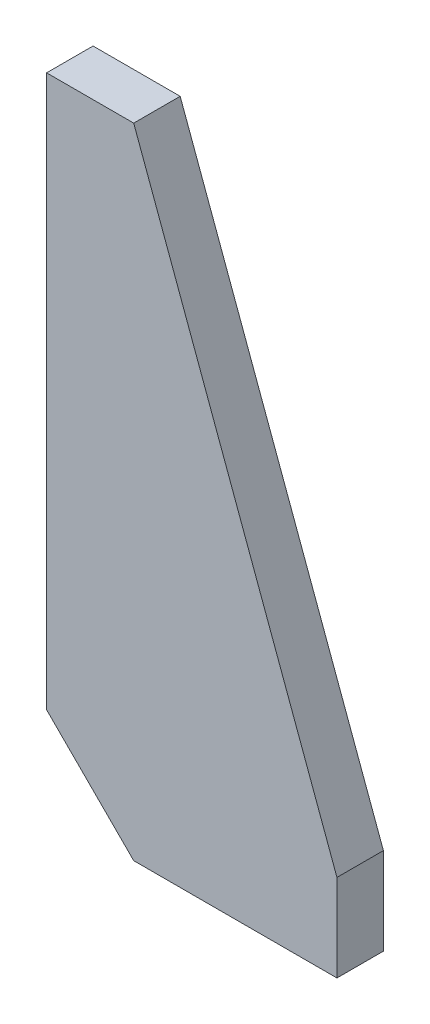
from build123d import *

# Parameters (mm, degrees)
BOSS_EXTRUDE1_DEPTH = 8
CHAMFER1_SIZE       = 15


with BuildPart() as part:
    # Sketch1 → Boss-Extrude1 (new body)
    with BuildSketch(Plane.XY):
        Polygon((0, 0), (50, 0), (50, 15), (15, 110), (0, 110), align=None)
    extrude(amount=BOSS_EXTRUDE1_DEPTH)

    # Chamfer1
    chamfer1_edges = [part.edges().sort_by_distance(p)[0] for p in [
        (0, 0, 4),
    ]]
    chamfer(chamfer1_edges, length=CHAMFER1_SIZE)


solid = part.part
